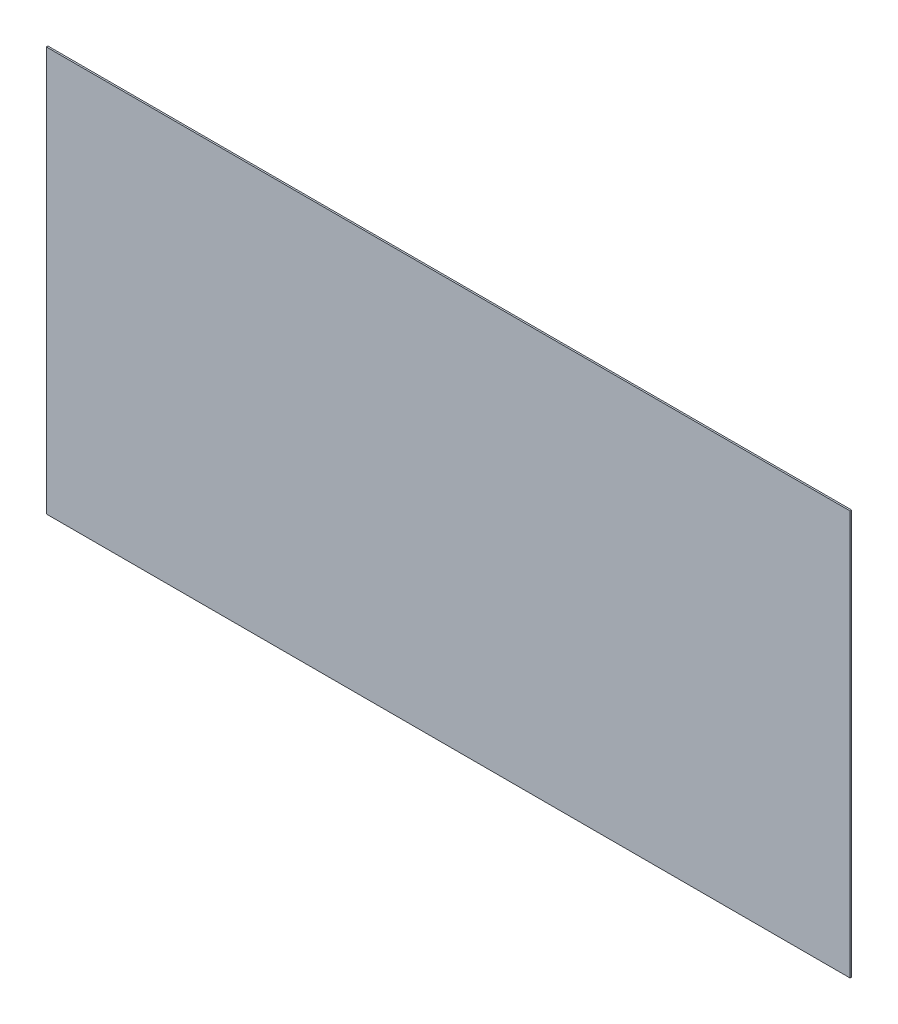
from build123d import *

# Parameters (mm, degrees)
SKETCH1_W           = 3000
SKETCH1_H           = 1510
BOSS_EXTRUDE1_DEPTH = 6


with BuildPart() as part:
    # Sketch1 → Boss-Extrude1 (new body)
    with BuildSketch(Plane.XY):
        with Locations((1500, 755)):
            Rectangle(SKETCH1_W, SKETCH1_H)
    extrude(amount=BOSS_EXTRUDE1_DEPTH)


solid = part.part
